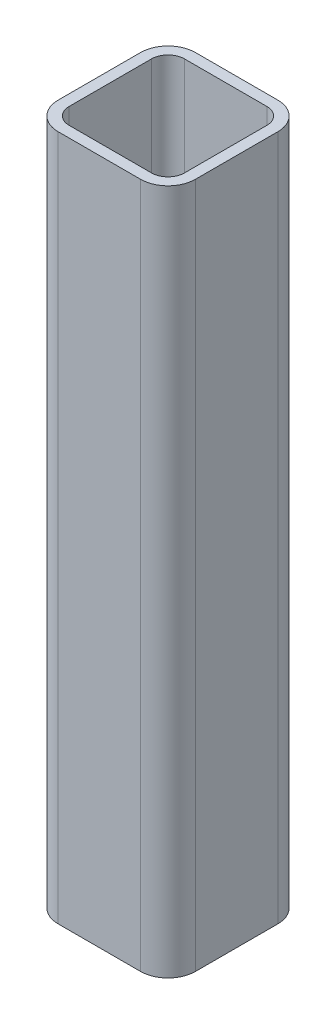
SolidWorks part; units mm, degrees
material "Q235B"
ref_plane "Front Plane" through (0, 0, 0) normal (0, 0, 1) x (1, 0, 0)
ref_plane "Top Plane" through (0, 0, 0) normal (0, 1, 0) x (1, 0, 0)
ref_plane "Right Plane" through (0, 0, 0) normal (1, 0, 0) x (0, 0, -1)
other "Configuration Table"
sketch "Sketch1" plane through (0, 0, 0) normal (0, 1, 0) x (1, 0, 0)
  line L0 (-15, 21) -> (15, 21)
  line L1 (-15, -25) -> (15, -25)
  line L2 (-25, -15) -> (-25, 15)
  line L3 (-15, 25) -> (15, 25)
  line L4 (25, -15) -> (25, 15)
  line L5 (-25, -25) -> (25, 25) construction
  line L6 (-25, 25) -> (25, -25) construction
  line L7 (21, -15) -> (21, 15)
  line L8 (-15, -21) -> (15, -21)
  line L9 (-21, -15) -> (-21, 15)
  arc A0 (15, -25) -> (25, -15) centre (15, -15) ccw
  arc A1 (15, 25) -> (25, 15) centre (15, 15) cw
  arc A2 (-25, 15) -> (-15, 25) centre (-15, 15) cw
  arc A3 (-15, -25) -> (-25, -15) centre (-15, -15) cw
  arc A4 (15, 21) -> (21, 15) centre (15, 15) cw
  arc A5 (15, -21) -> (21, -15) centre (15, -15) ccw
  arc A6 (-15, -21) -> (-21, -15) centre (-15, -15) cw
  arc A7 (-21, 15) -> (-15, 21) centre (-15, 15) cw
  point P0 (0, 0)
  dimension "D2" = 10
  dimension "D3" = 10
  dimension "D1" = 50
  dimension "D4" = 4
extrude "Boss-Extrude1" add sketch "Sketch1" along normal blind 250
